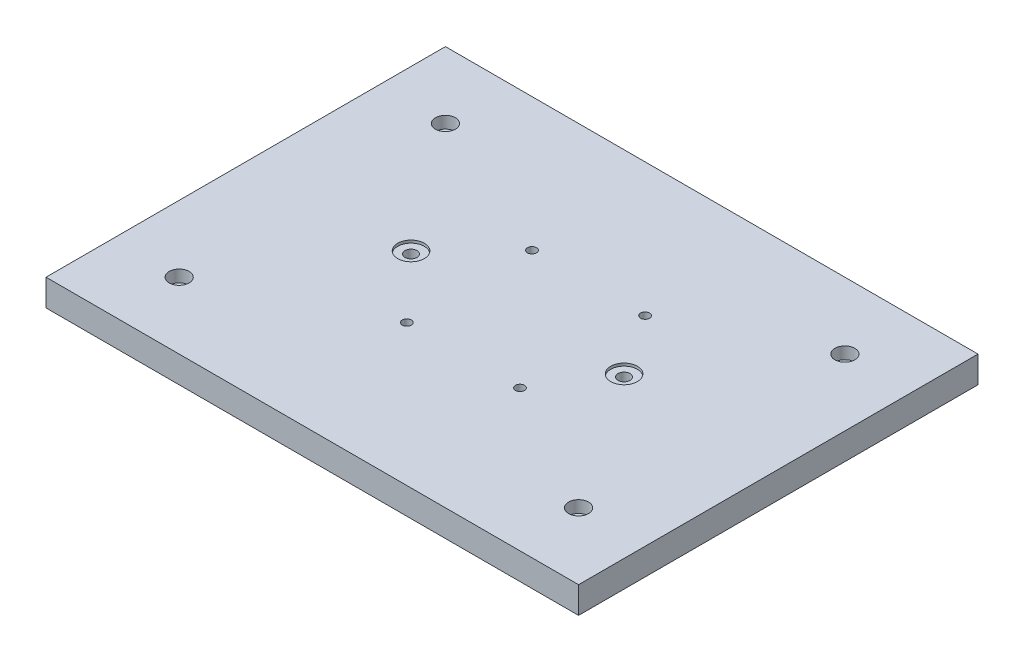
SolidWorks part; units mm, degrees
ref_plane "Front Plane" through (0, 0, 0) normal (0, 0, 1) x (1, 0, 0)
ref_plane "Top Plane" through (0, 0, 0) normal (0, 1, 0) x (1, 0, 0)
ref_plane "Right Plane" through (0, 0, 0) normal (1, 0, 0) x (0, 0, -1)
sketch "Sketch1" plane through (0, 0, 0) normal (0, 1, 0) x (1, 0, 0)
  line L1 (-200, 150) -> (200, 150)
  line L2 (-200, 150) -> (-200, -150)
  line L3 (-200, -150) -> (200, -150)
  line L4 (200, 150) -> (200, -150)
  line L5 (-200, 150) -> (200, -150) construction
  line L6 (-200, -150) -> (200, 150) construction
  point P0 (0, 0)
  dimension "D1" = 400
  dimension "D2" = 300
extrude "Boss-Extrude1" add sketch "Sketch1" along normal blind 20
sketch "Sketch2" plane through (0, 20, 0) normal (0, 1, 0) x (1, 0, 0)
  line L1 (-150, -100) -> (150, -100)
  line L2 (-150, -100) -> (-150, 100)
  line L3 (-150, 100) -> (150, 100)
  line L4 (150, -100) -> (150, 100)
  line L5 (-150, -100) -> (150, 100) construction
  line L6 (-150, 100) -> (150, -100) construction
  point P0 (0, 0)
  dimension "D1" = 300
  dimension "D2" = 200
hole_wizard "Hole size per socket head cap screw type1" positions "Sketch3" profile "Sketch4" counterbore size "M8" standard "GB" end condition through all
sketch "Sketch3" plane through (0, 20, 0) normal (0, 1, 0) x (1, 0, 0)
  point P0 (-150, 100)
  point P3 (-150, -100)
  point P6 (150, 100)
  point P9 (150, -100)
sketch "Sketch4" plane through (-150, 20, -100) normal (1, 0, 0) x (0, 0, 1)
  line L0 (0, 0) -> (0, 20)
  line L1 (0, 20) -> (4.5, 20)
  line L3 (4.5, 20) -> (4.5, 9)
  line L4 (4.5, 9) -> (7.5, 9)
  line L5 (7.5, 9) -> (7.5, 0)
  line L7 (7.5, 0) -> (0, 0)
  line L11 (0, -6.35) -> (0, 107.95) construction
  dimension "通孔孔直径" = 9
  dimension "通孔孔深度" = 20
  dimension "柱形沉头孔直径" = 15
  dimension "柱形沉头孔深度" = 9
sketch "Sketch5" plane through (0, 20, 0) normal (0, 1, 0) x (1, 0, 0)
  circle A0 centre (-80, 4.1664) radius 10
  circle A1 centre (80, 4.1664) radius 10
  dimension "D1" = 20
extrude "Cut-Extrude1" cut sketch "Sketch5" against normal blind 2
hole_wizard "Hole size per socket head cap screw type2" positions "Sketch6" profile "Sketch7" counterbore size "M8" standard "GB" end condition through all
sketch "Sketch6" plane through (0, 0, 0) normal (0, -1, 0) x (-1, 0, 0)
  point P0 (80, 4.1664)
  point P3 (-80, 4.1664)
sketch "Sketch7" plane through (-80, 0, -4.1664) normal (1, 0, 0) x (0, 0, -1)
  line L0 (0, 0) -> (0, 20)
  line L1 (0, 20) -> (4.5, 20)
  line L3 (4.5, 20) -> (4.5, 9)
  line L4 (4.5, 9) -> (7.5, 9)
  line L5 (7.5, 9) -> (7.5, 0)
  line L7 (7.5, 0) -> (0, 0)
  line L11 (0, -6.35) -> (0, 107.95) construction
  dimension "通孔孔直径" = 9
  dimension "通孔孔深度" = 20
  dimension "柱形沉头孔直径" = 15
  dimension "柱形沉头孔深度" = 9
sketch "Sketch8" plane through (0, 20, 0) normal (0, 1, 0) x (1, 0, 0)
  line L0 (200, -150) -> (200, 150) construction
  line L1 (-35, 50) -> (50, 50) construction
  line L2 (-35, 50) -> (-35, -44) construction
  line L3 (-35, -44) -> (50, -44) construction
  line L4 (50, 50) -> (50, -44) construction
  line L5 (200, 150) -> (-200, 150) construction
  dimension "D1" = 85
  dimension "D2" = 94
  dimension "D3" = 150
  dimension "D4" = 100
hole_wizard "M8 Tapped Hole1" positions "Sketch9" profile "Sketch10" tap size "M8" standard "GB" end condition through all
sketch "Sketch9" plane through (0, 20, 0) normal (0, 1, 0) x (1, 0, 0)
  point P0 (-35, 50)
  point P3 (-35, -44)
  point P5 (50, -44)
  point P8 (50, 50)
sketch "Sketch10" plane through (-35, 20, -50) normal (1, 0, 0) x (0, 0, 1)
  line L0 (0, 0) -> (0, 20)
  line L1 (0, 20) -> (3.4, 20)
  line L2 (3.4, 20) -> (3.4, 0)
  line L5 (3.4, 0) -> (0, 0)
  line L11 (0, -6.35) -> (0, 107.95) construction
  dimension "通孔螺纹孔钻头直径" = 6.8
  dimension "通孔螺纹孔钻头深度" = 20
cosmetic thread "Cosmetic Thread1"
cosmetic thread "Cosmetic Thread2"
cosmetic thread "Cosmetic Thread3"
cosmetic thread "Cosmetic Thread4"
